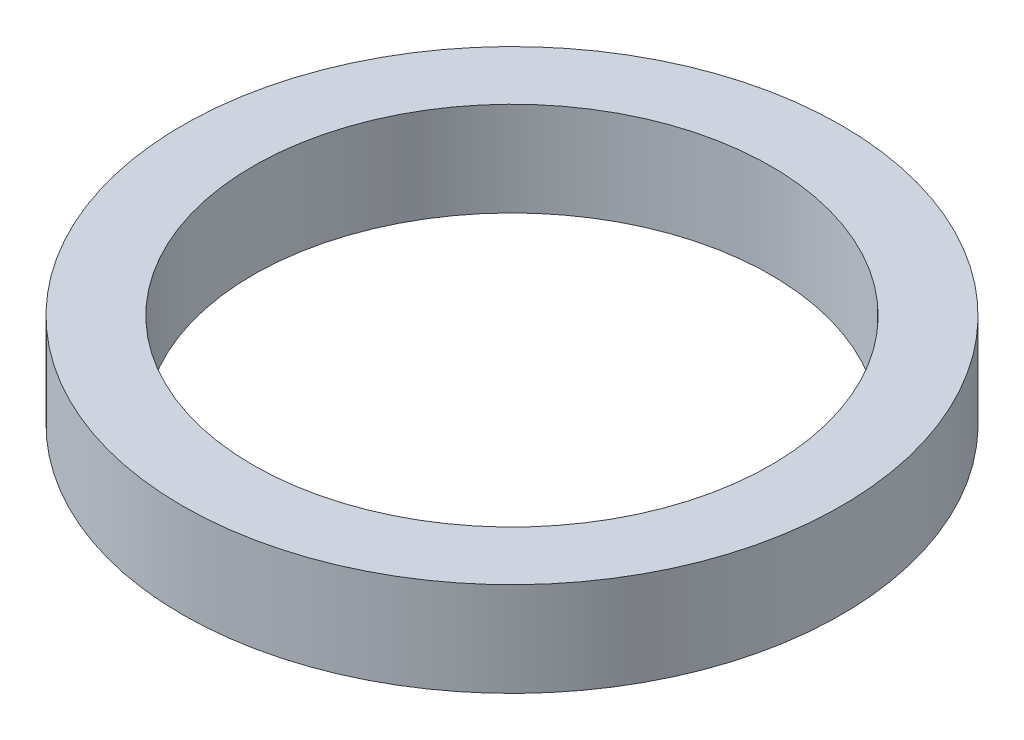
SolidWorks part; units mm, degrees
ref_plane "Front Plane" through (0, 0, 0) normal (0, 0, 1) x (1, 0, 0)
ref_plane "Top Plane" through (0, 0, 0) normal (0, 1, 0) x (1, 0, 0)
ref_plane "Right Plane" through (0, 0, 0) normal (1, 0, 0) x (0, 0, -1)
other "Configuration Table"
sketch "Sketch1" plane through (0, 0, 0) normal (0, 1, 0) x (1, 0, 0)
  circle A0 centre (0, 0) radius 7
  circle A1 centre (0, 0) radius 5.5
  dimension "D1" = 14
  dimension "D2" = 11
extrude "Boss-Extrude1" add sketch "Sketch1" along normal mid plane 2
